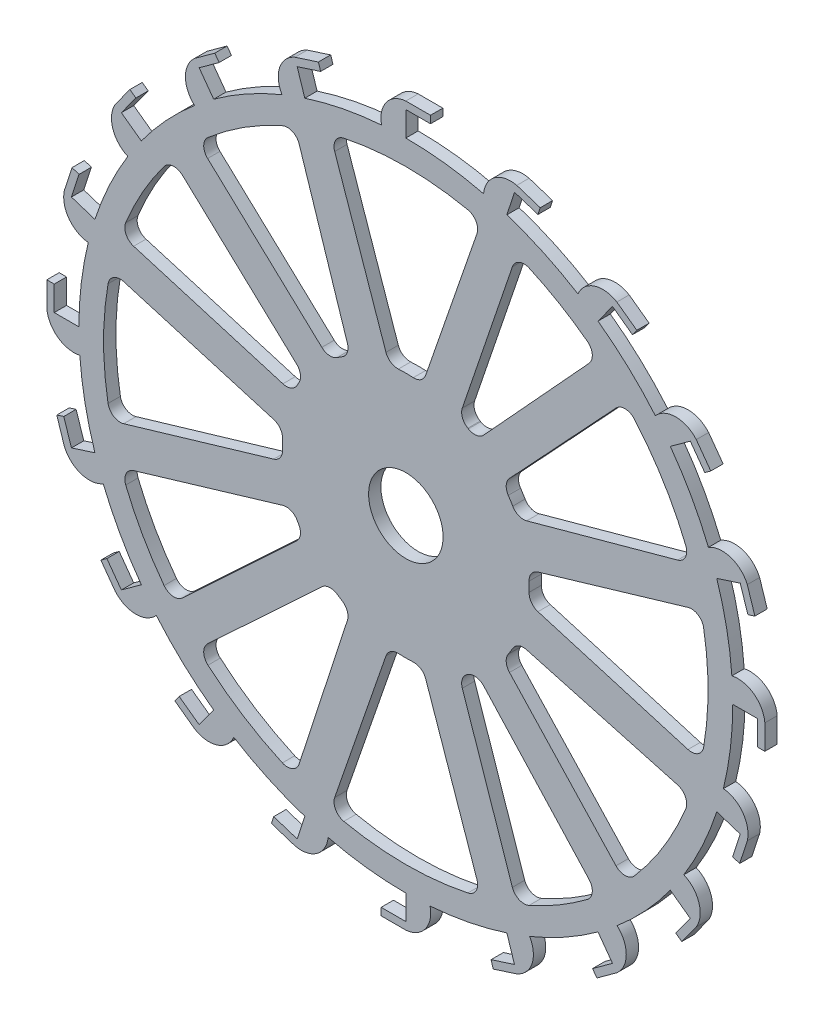
from build123d import *

# Parameters (mm, degrees)
SKETCH_1_R          = 15
EXTRUDE_1_DEPTH     = 5
EXTRUDE_2_DEPTH     = 5
FILLET_1_R          = 5
SKETCH_4_R          = 15.1
SKETCH_4_R_2        = 15
CUT_EXTRUDE_1_DEPTH = 206.828812366


with BuildPart() as part:
    # 草图1 → 凸台-拉伸1 (new body)
    with BuildSketch(Plane.XY):
        with BuildLine():
            Line((0, 145.5), (10, 145.5))
            Line((10, 145.5), (10, 142.5))
            Line((10, 142.5), (0, 142.5))
            Line((0, 142.5), (0, 132.5))
            ThreePointArc((0, 132.5), (15.863549131, 131.546941466), (31.498888588, 128.701476362))
            ThreePointArc((31.498888588, 128.701476362), (36.030071565, 136.601261654), (44.961972682, 138.378723121))
            Line((44.961972682, 138.378723121), (54.472537845, 135.288553177))
            Line((54.472537845, 135.288553177), (53.545486861, 132.435383628))
            Line((53.545486861, 132.435383628), (44.034921698, 135.525553572))
            Line((44.034921698, 135.525553572), (40.944751755, 126.014988409))
            ThreePointArc((40.944751755, 126.014988409), (55.737372243, 120.206469607), (69.728166645, 112.668685873))
            ThreePointArc((69.728166645, 112.668685873), (76.478745648, 118.781615608), (85.522754209, 117.711972682))
            Line((85.522754209, 117.711972682), (93.612924152, 111.834120159))
            Line((93.612924152, 111.834120159), (91.849568395, 109.407069176))
            Line((91.849568395, 109.407069176), (83.759398452, 115.284921698))
            Line((83.759398452, 115.284921698), (77.881545929, 107.194751755))
            ThreePointArc((77.881545929, 107.194751755), (90.155233016, 97.099350976), (101.131965925, 85.607099402))
            ThreePointArc((101.131965925, 85.607099402), (109.441147249, 89.334797426), (117.711972682, 85.522754209))
            Line((117.711972682, 85.522754209), (123.589825204, 77.432584265))
            Line((123.589825204, 77.432584265), (121.162774221, 75.669228508))
            Line((121.162774221, 75.669228508), (115.284921698, 83.759398452))
            Line((115.284921698, 83.759398452), (107.194751755, 77.881545929))
            ThreePointArc((107.194751755, 77.881545929), (115.748071432, 64.48747134), (122.636263754, 50.165693582))
            ThreePointArc((122.636263754, 50.165693582), (131.690686836, 51.14326684), (138.378723121, 44.961972682))
            Line((138.378723121, 44.961972682), (141.468893065, 35.451407519))
            Line((141.468893065, 35.451407519), (138.615723516, 34.524356535))
            Line((138.615723516, 34.524356535), (135.525553572, 44.034921698))
            Line((135.525553572, 44.034921698), (126.014988409, 40.944751755))
            ThreePointArc((126.014988409, 40.944751755), (130.010682152, 25.563108698), (132.136069628, 9.813720149))
            ThreePointArc((132.136069628, 9.813720149), (141.049424452, 7.94547696), (145.5, 0))
            Line((145.5, 0), (145.5, -10))
            Line((145.5, -10), (142.5, -10))
            Line((142.5, -10), (142.5, 0))
            Line((142.5, 0), (132.5, 0))
            ThreePointArc((132.5, 0), (131.546941466, -15.863549131), (128.701476362, -31.498888588))
            ThreePointArc((128.701476362, -31.498888588), (136.601261654, -36.030071565), (138.378723121, -44.961972682))
            Line((138.378723121, -44.961972682), (135.288553177, -54.472537845))
            Line((135.288553177, -54.472537845), (132.435383628, -53.545486861))
            Line((132.435383628, -53.545486861), (135.525553572, -44.034921698))
            Line((135.525553572, -44.034921698), (126.014988409, -40.944751755))
            ThreePointArc((126.014988409, -40.944751755), (120.206469607, -55.737372243), (112.668685873, -69.728166645))
            ThreePointArc((112.668685873, -69.728166645), (118.781615608, -76.478745648), (117.711972682, -85.522754209))
            Line((117.711972682, -85.522754209), (111.834120159, -93.612924152))
            Line((111.834120159, -93.612924152), (109.407069176, -91.849568395))
            Line((109.407069176, -91.849568395), (115.284921698, -83.759398452))
            Line((115.284921698, -83.759398452), (107.194751755, -77.881545929))
            ThreePointArc((107.194751755, -77.881545929), (97.099350976, -90.155233016), (85.607099402, -101.131965925))
            ThreePointArc((85.607099402, -101.131965925), (89.334797426, -109.441147249), (85.522754209, -117.711972682))
            Line((85.522754209, -117.711972682), (77.432584265, -123.589825204))
            Line((77.432584265, -123.589825204), (75.669228508, -121.162774221))
            Line((75.669228508, -121.162774221), (83.759398452, -115.284921698))
            Line((83.759398452, -115.284921698), (77.881545929, -107.194751755))
            ThreePointArc((77.881545929, -107.194751755), (64.48747134, -115.748071432), (50.165693582, -122.636263754))
            ThreePointArc((50.165693582, -122.636263754), (51.14326684, -131.690686836), (44.961972682, -138.378723121))
            Line((44.961972682, -138.378723121), (35.451407519, -141.468893065))
            Line((35.451407519, -141.468893065), (34.524356535, -138.615723516))
            Line((34.524356535, -138.615723516), (44.034921698, -135.525553572))
            Line((44.034921698, -135.525553572), (40.944751755, -126.014988409))
            ThreePointArc((40.944751755, -126.014988409), (25.563108698, -130.010682152), (9.813720149, -132.136069628))
            ThreePointArc((9.813720149, -132.136069628), (7.94547696, -141.049424452), (0, -145.5))
            Line((0, -145.5), (-10, -145.5))
            Line((-10, -145.5), (-10, -142.5))
            Line((-10, -142.5), (0, -142.5))
            Line((0, -142.5), (0, -132.5))
            ThreePointArc((0, -132.5), (-15.863549131, -131.546941466), (-31.498888588, -128.701476362))
            ThreePointArc((-31.498888588, -128.701476362), (-36.030071565, -136.601261654), (-44.961972682, -138.378723121))
            Line((-44.961972682, -138.378723121), (-54.472537845, -135.288553177))
            Line((-54.472537845, -135.288553177), (-53.545486861, -132.435383628))
            Line((-53.545486861, -132.435383628), (-44.034921698, -135.525553572))
            Line((-44.034921698, -135.525553572), (-40.944751755, -126.014988409))
            ThreePointArc((-40.944751755, -126.014988409), (-55.737372243, -120.206469607), (-69.728166645, -112.668685873))
            ThreePointArc((-69.728166645, -112.668685873), (-76.478745648, -118.781615608), (-85.522754209, -117.711972682))
            Line((-85.522754209, -117.711972682), (-93.612924152, -111.834120159))
            Line((-93.612924152, -111.834120159), (-91.849568395, -109.407069176))
            Line((-91.849568395, -109.407069176), (-83.759398452, -115.284921698))
            Line((-83.759398452, -115.284921698), (-77.881545929, -107.194751755))
            ThreePointArc((-77.881545929, -107.194751755), (-90.155233016, -97.099350976), (-101.131965925, -85.607099402))
            ThreePointArc((-101.131965925, -85.607099402), (-109.441147249, -89.334797426), (-117.711972682, -85.522754209))
            Line((-117.711972682, -85.522754209), (-123.589825204, -77.432584265))
            Line((-123.589825204, -77.432584265), (-121.162774221, -75.669228508))
            Line((-121.162774221, -75.669228508), (-115.284921698, -83.759398452))
            Line((-115.284921698, -83.759398452), (-107.194751755, -77.881545929))
            ThreePointArc((-107.194751755, -77.881545929), (-115.748071432, -64.48747134), (-122.636263754, -50.165693582))
            ThreePointArc((-122.636263754, -50.165693582), (-131.690686836, -51.14326684), (-138.378723121, -44.961972682))
            Line((-138.378723121, -44.961972682), (-141.468893065, -35.451407519))
            Line((-141.468893065, -35.451407519), (-138.615723516, -34.524356535))
            Line((-138.615723516, -34.524356535), (-135.525553572, -44.034921698))
            Line((-135.525553572, -44.034921698), (-126.014988409, -40.944751755))
            ThreePointArc((-126.014988409, -40.944751755), (-130.010682152, -25.563108698), (-132.136069628, -9.813720149))
            ThreePointArc((-132.136069628, -9.813720149), (-141.049424452, -7.94547696), (-145.5, 0))
            Line((-145.5, 0), (-145.5, 10))
            Line((-145.5, 10), (-142.5, 10))
            Line((-142.5, 10), (-142.5, 0))
            Line((-142.5, 0), (-132.5, 0))
            ThreePointArc((-132.5, 0), (-131.546941466, 15.863549131), (-128.701476362, 31.498888588))
            ThreePointArc((-128.701476362, 31.498888588), (-136.601261654, 36.030071565), (-138.378723121, 44.961972682))
            Line((-138.378723121, 44.961972682), (-135.288553177, 54.472537845))
            Line((-135.288553177, 54.472537845), (-132.435383628, 53.545486861))
            Line((-132.435383628, 53.545486861), (-135.525553572, 44.034921698))
            Line((-135.525553572, 44.034921698), (-126.014988409, 40.944751755))
            ThreePointArc((-126.014988409, 40.944751755), (-120.206469607, 55.737372243), (-112.668685873, 69.728166645))
            ThreePointArc((-112.668685873, 69.728166645), (-118.781615608, 76.478745648), (-117.711972682, 85.522754209))
            Line((-117.711972682, 85.522754209), (-111.834120159, 93.612924152))
            Line((-111.834120159, 93.612924152), (-109.407069176, 91.849568395))
            Line((-109.407069176, 91.849568395), (-115.284921698, 83.759398452))
            Line((-115.284921698, 83.759398452), (-107.194751755, 77.881545929))
            ThreePointArc((-107.194751755, 77.881545929), (-97.099350976, 90.155233016), (-85.607099402, 101.131965925))
            ThreePointArc((-85.607099402, 101.131965925), (-89.334797426, 109.441147249), (-85.522754209, 117.711972682))
            Line((-85.522754209, 117.711972682), (-77.432584265, 123.589825204))
            Line((-77.432584265, 123.589825204), (-75.669228508, 121.162774221))
            Line((-75.669228508, 121.162774221), (-83.759398452, 115.284921698))
            Line((-83.759398452, 115.284921698), (-77.881545929, 107.194751755))
            ThreePointArc((-77.881545929, 107.194751755), (-64.48747134, 115.748071432), (-50.165693582, 122.636263754))
            ThreePointArc((-50.165693582, 122.636263754), (-51.14326684, 131.690686836), (-44.961972682, 138.378723121))
            Line((-44.961972682, 138.378723121), (-35.451407519, 141.468893065))
            Line((-35.451407519, 141.468893065), (-34.524356535, 138.615723516))
            Line((-34.524356535, 138.615723516), (-44.034921698, 135.525553572))
            Line((-44.034921698, 135.525553572), (-40.944751755, 126.014988409))
            ThreePointArc((-40.944751755, 126.014988409), (-25.563108698, 130.010682152), (-9.813720149, 132.136069628))
            ThreePointArc((-9.813720149, 132.136069628), (-7.94547696, 141.049424452), (0, 145.5))
        make_face()
        Circle(SKETCH_1_R, mode=Mode.SUBTRACT)
        with BuildLine():
            Line((115.4655256, -40.91408557), (25.295414942, -16.128917599))
            Line((25.295414942, -16.128917599), (88.873223604, -84.30777026))
            ThreePointArc((88.873223604, -84.30777026), (104.447757632, -64.00715527), (115.4655256, -40.91408557))
        make_face(mode=Mode.SUBTRACT)
        with BuildLine():
            Line((-30.646438581, 118.604577493), (0, 30))
            Line((0, 30), (30.646438581, 118.604577493))
            ThreePointArc((30.646438581, 118.604577493), (0, 122.5), (-30.646438581, 118.604577493))
        make_face(mode=Mode.SUBTRACT)
        with BuildLine():
            Line((-119.601341953, -26.490923031), (-30, 0))
            Line((-30, 0), (-119.601341953, 26.490923031))
            ThreePointArc((-119.601341953, 26.490923031), (-122.5, 0), (-119.601341953, -26.490923031))
        make_face(mode=Mode.SUBTRACT)
        with BuildLine():
            Line((30.646438581, -118.604577493), (0, -30))
            Line((0, -30), (-30.646438581, -118.604577493))
            ThreePointArc((-30.646438581, -118.604577493), (0, -122.5), (30.646438581, -118.604577493))
        make_face(mode=Mode.SUBTRACT)
        with BuildLine():
            Line((-115.467174059, 40.909433079), (-26.347643759, 14.345789221))
            Line((-26.347643759, 14.345789221), (-94.537709943, 77.902961425))
            ThreePointArc((-94.537709943, 77.902961425), (-106.619149832, 60.320866116), (-115.467174059, 40.909433079))
        make_face(mode=Mode.SUBTRACT)
        with BuildLine():
            Line((-94.537709943, -77.902961425), (-26.347643759, -14.345789221))
            Line((-26.347643759, -14.345789221), (-115.467174059, -40.909433079))
            ThreePointArc((-115.467174059, -40.909433079), (-106.619149832, -60.320866116), (-94.537709943, -77.902961425))
        make_face(mode=Mode.SUBTRACT)
        with BuildLine():
            Line((-44.916491293, -113.968235969), (-16.109056419, -25.308067909))
            Line((-16.109056419, -25.308067909), (-84.307729511, -88.87326226))
            ThreePointArc((-84.307729511, -88.87326226), (-65.819178337, -103.315467201), (-44.916491293, -113.968235969))
        make_face(mode=Mode.SUBTRACT)
        with BuildLine():
            Line((77.904348966, -94.536566535), (15, -25.980762114))
            Line((15, -25.980762114), (44.913590331, -113.969379237))
            ThreePointArc((44.913590331, -113.969379237), (62.172904916, -105.549892915), (77.904348966, -94.536566535))
        make_face(mode=Mode.SUBTRACT)
        with BuildLine():
            Line((88.873223604, 84.30777026), (25.295414942, 16.128917599))
            Line((25.295414942, 16.128917599), (115.4655256, 40.91408557))
            ThreePointArc((115.4655256, 40.91408557), (104.447757632, 64.00715527), (88.873223604, 84.30777026))
        make_face(mode=Mode.SUBTRACT)
        with BuildLine():
            Line((119.601341953, 26.490923031), (30, 0))
            Line((30, 0), (119.601341953, -26.490923031))
            ThreePointArc((119.601341953, -26.490923031), (122.5, 0), (119.601341953, 26.490923031))
        make_face(mode=Mode.SUBTRACT)
        with BuildLine():
            Line((44.913590331, 113.969379237), (15, 25.980762114))
            Line((15, 25.980762114), (77.904348966, 94.536566535))
            ThreePointArc((77.904348966, 94.536566535), (62.172904916, 105.549892915), (44.913590331, 113.969379237))
        make_face(mode=Mode.SUBTRACT)
        with BuildLine():
            Line((-84.307729511, 88.87326226), (-16.109056419, 25.308067909))
            Line((-16.109056419, 25.308067909), (-44.916491293, 113.968235969))
            ThreePointArc((-44.916491293, 113.968235969), (-65.819178337, 103.315467201), (-84.307729511, 88.87326226))
        make_face(mode=Mode.SUBTRACT)
    extrude(amount=EXTRUDE_1_DEPTH)

    # 草图3 → 凸台-拉伸2 (add, through all)
    with BuildSketch(Plane(origin=(0, 0, 0), x_dir=(-1, 0, 0), z_dir=(0, 0, -1))):
        with BuildLine():
            Line((-25.295414942, -16.128917599), (-45.105993407, -21.574275393))
            ThreePointArc((-45.105993407, -21.574275393), (-42.417440133, -26.471886457), (-39.199264179, -31.03897047))
            Line((-39.199264179, -31.03897047), (-25.295414942, -16.128917599))
        make_face()
        with BuildLine():
            Line((0, 30), (6.758841971, 49.541074425))
            ThreePointArc((6.758841971, 49.541074425), (0, 50), (-6.758841971, 49.541074425))
            Line((-6.758841971, 49.541074425), (0, 30))
        make_face()
        with BuildLine():
            Line((30, 0), (49.66096107, -5.812825958))
            ThreePointArc((49.66096107, -5.812825958), (50, 0), (49.66096107, 5.812825958))
            Line((49.66096107, 5.812825958), (30, 0))
        make_face()
        with BuildLine():
            Line((0, -30), (-6.758841971, -49.541074425))
            ThreePointArc((-6.758841971, -49.541074425), (0, -50), (6.758841971, -49.541074425))
            Line((6.758841971, -49.541074425), (0, -30))
        make_face()
        with BuildLine():
            Line((26.347643759, 14.345789221), (45.767009048, 20.134072684))
            ThreePointArc((45.767009048, 20.134072684), (43.701412136, 24.293755933), (41.258765465, 28.243836005))
            Line((41.258765465, 28.243836005), (26.347643759, 14.345789221))
        make_face()
        with BuildLine():
            Line((26.347643759, -14.345789221), (41.258765465, -28.243836005))
            ThreePointArc((41.258765465, -28.243836005), (43.701412136, -24.293755933), (45.767009048, -20.134072684))
            Line((45.767009048, -20.134072684), (26.347643759, -14.345789221))
        make_face()
        with BuildLine():
            Line((16.109056419, -25.308067909), (22.408962626, -44.697185527))
            ThreePointArc((22.408962626, -44.697185527), (26.857377053, -42.174415205), (31.024833654, -39.210453921))
            Line((31.024833654, -39.210453921), (16.109056419, -25.308067909))
        make_face()
        with BuildLine():
            Line((-15, -25.980762114), (-28.717400548, -40.930562002))
            ThreePointArc((-28.717400548, -40.930562002), (-25.202615525, -43.183656292), (-21.512116377, -45.13567158))
            Line((-21.512116377, -45.13567158), (-15, -25.980762114))
        make_face()
        with BuildLine():
            Line((-25.295414942, 16.128917599), (-39.199264179, 31.03897047))
            ThreePointArc((-39.199264179, 31.03897047), (-42.417440133, 26.471886457), (-45.105993407, 21.574275393))
            Line((-45.105993407, 21.574275393), (-25.295414942, 16.128917599))
        make_face()
        with BuildLine():
            Line((-30, 0), (-49.66096107, 5.812825958))
            ThreePointArc((-49.66096107, 5.812825958), (-50, 0), (-49.66096107, -5.812825958))
            Line((-49.66096107, -5.812825958), (-30, 0))
        make_face()
        with BuildLine():
            Line((-15, 25.980762114), (-21.512116377, 45.13567158))
            ThreePointArc((-21.512116377, 45.13567158), (-25.202615525, 43.183656292), (-28.717400548, 40.930562002))
            Line((-28.717400548, 40.930562002), (-15, 25.980762114))
        make_face()
        with BuildLine():
            Line((16.109056419, 25.308067909), (31.024833654, 39.210453921))
            ThreePointArc((31.024833654, 39.210453921), (26.857377053, 42.174415205), (22.408962626, 44.697185527))
            Line((22.408962626, 44.697185527), (16.109056419, 25.308067909))
        make_face()
    extrude(amount=-EXTRUDE_2_DEPTH)

    # 圆角1
    fillet_1_edges = [part.edges().sort_by_distance(p)[0] for p in [
        (88.873223604, -84.30777026, 2.5),
        (115.4655256, -40.91408557, 2.5),
        (30.646438581, 118.604577493, 2.5),
        (-30.646438581, 118.604577493, 2.5),
        (-119.601341953, 26.490923031, 2.5),
        (-119.601341953, -26.490923031, 2.5),
        (-30.646438581, -118.604577493, 2.5),
        (30.646438581, -118.604577493, 2.5),
        (-94.537709943, 77.902961425, 2.5),
        (-115.467174059, 40.909433079, 2.5),
        (-115.467174059, -40.909433079, 2.5),
        (-94.537709943, -77.902961425, 2.5),
        (-84.307729511, -88.87326226, 2.5),
        (-44.916491293, -113.968235969, 2.5),
        (44.913590331, -113.969379237, 2.5),
        (77.904348966, -94.536566535, 2.5),
        (115.4655256, 40.91408557, 2.5),
        (88.873223604, 84.30777026, 2.5),
        (119.601341953, -26.490923031, 2.5),
        (119.601341953, 26.490923031, 2.5),
        (77.904348966, 94.536566535, 2.5),
        (44.913590331, 113.969379237, 2.5),
        (-44.916491293, 113.968235969, 2.5),
        (-84.307729511, 88.87326226, 2.5),
        (39.199264179, -31.03897047, 2.5),
        (45.105993407, -21.574275393, 2.5),
        (6.758841971, 49.541074425, 2.5),
        (-6.758841971, 49.541074425, 2.5),
        (-49.66096107, 5.812825958, 2.5),
        (-49.66096107, -5.812825958, 2.5),
        (-6.758841971, -49.541074425, 2.5),
        (6.758841971, -49.541074425, 2.5),
        (-41.258765465, 28.243836005, 2.5),
        (-45.767009048, 20.134072684, 2.5),
        (-45.767009048, -20.134072684, 2.5),
        (-41.258765465, -28.243836005, 2.5),
        (-31.024833654, -39.210453921, 2.5),
        (-22.408962626, -44.697185527, 2.5),
        (21.512116377, -45.13567158, 2.5),
        (28.717400548, -40.930562002, 2.5),
        (45.105993407, 21.574275393, 2.5),
        (39.199264179, 31.03897047, 2.5),
        (49.66096107, -5.812825958, 2.5),
        (49.66096107, 5.812825958, 2.5),
        (28.717400548, 40.930562002, 2.5),
        (21.512116377, 45.13567158, 2.5),
        (-22.408962626, 44.697185527, 2.5),
        (-31.024833654, 39.210453921, 2.5),
    ]]
    fillet(fillet_1_edges, radius=FILLET_1_R)

    # 草图4 → 切除-拉伸1 (cut, through all)
    with BuildSketch(Plane(origin=(0, 0, 0), x_dir=(-1, 0, 0), z_dir=(0, 0, -1))):
        Circle(SKETCH_4_R)
        Circle(SKETCH_4_R_2, mode=Mode.SUBTRACT)
    extrude(amount=-CUT_EXTRUDE_1_DEPTH, mode=Mode.SUBTRACT)


solid = part.part
